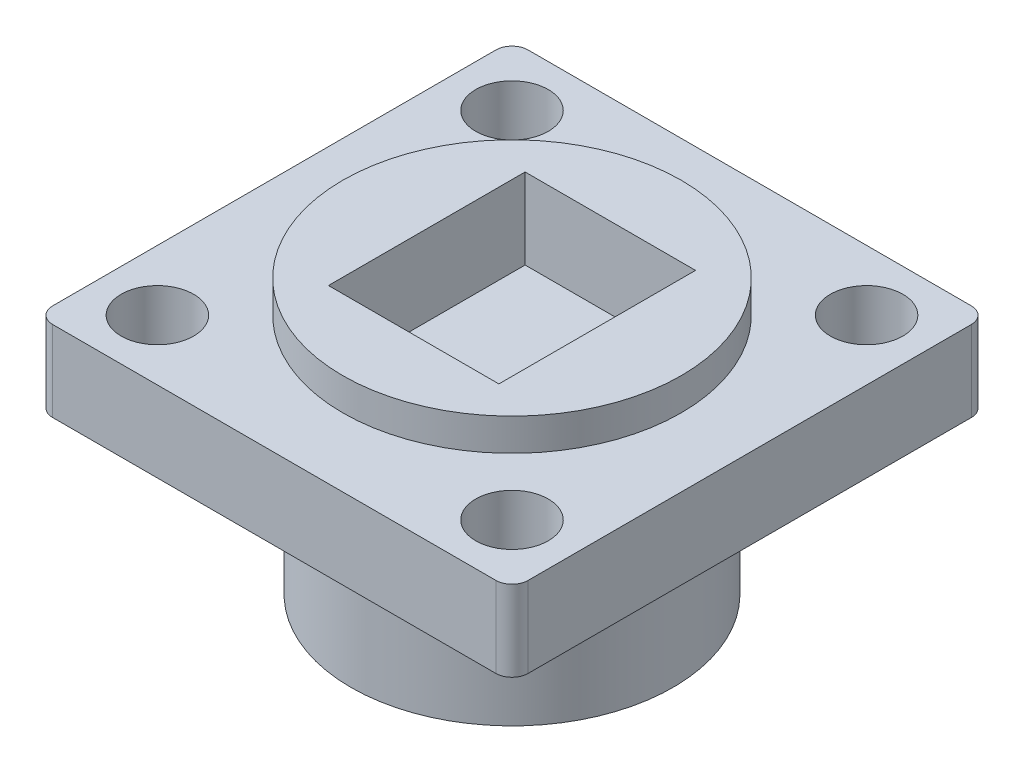
SolidWorks part; units mm, degrees
ref_plane "前视基准面" through (0, 0, 0) normal (0, 0, 1) x (1, 0, 0)
ref_plane "上视基准面" through (0, 0, 0) normal (0, 1, 0) x (1, 0, 0)
ref_plane "右视基准面" through (0, 0, 0) normal (1, 0, 0) x (0, 0, -1)
sketch "草图1" plane through (0, 0, 0) normal (0, 1, 0) x (1, 0, 0)
  circle A0 centre (0, 0) radius 10
  dimension "D1" = 20
extrude "凸台-拉伸1" add sketch "草图1" along normal blind 10
sketch "草图2" plane through (0, 10, 0) normal (0, 1, 0) x (1, 0, 0)
  line L1 (-14.75, 14.75) -> (14.75, 14.75)
  line L2 (-14.75, 14.75) -> (-14.75, -14.75)
  line L3 (-14.75, -14.75) -> (14.75, -14.75)
  line L4 (14.75, 14.75) -> (14.75, -14.75)
  line L5 (-14.75, 14.75) -> (14.75, -14.75) construction
  line L6 (-14.75, -14.75) -> (14.75, 14.75) construction
  point P0 (0, 0)
  dimension "D1" = 29.5
extrude "凸台-拉伸2" add sketch "草图2" along normal blind 5
sketch "草图3" plane through (0, 15, 0) normal (0, 1, 0) x (1, 0, 0)
  circle A0 centre (0, 0) radius 10.5
  dimension "D1" = 21
extrude "凸台-拉伸3" add sketch "草图3" along normal blind 17
sketch "草图4" plane through (0, 15, 0) normal (0, 1, 0) x (1, 0, 0)
  line L1 (-11, 11) -> (11, 11) construction
  line L2 (-11, 11) -> (-11, -11) construction
  line L3 (-11, -11) -> (11, -11) construction
  line L4 (11, 11) -> (11, -11) construction
  line L5 (-11, 11) -> (11, -11) construction
  line L6 (-11, -11) -> (11, 11) construction
  circle A0 centre (11, 11) radius 2.25
  circle A1 centre (-11, 11) radius 2.25
  circle A2 centre (-11, -11) radius 2.25
  circle A3 centre (11, -11) radius 2.25
  point P0 (0, 0)
  dimension "D2" = 4.5
  dimension "D1" = 22
extrude "切除-拉伸1" cut sketch "草图4" against normal blind 17
fillet "圆角1" radius 1 4 edges at (-14.75, 12.5, -14.75) (14.75, 12.5, -14.75) (14.75, 12.5, 14.75) (-14.75, 12.5, 14.75)
sketch "草图5" plane through (0, 32, 0) normal (0, 1, 0) x (1, 0, 0)
  circle A1 centre (0, 0) radius 10.5
  circle A2 centre (0, 0) radius 10.5
  dimension "D1" = 0
extrude "切除-拉伸2" cut sketch "草图5" against normal blind 15
sketch "草图6" plane through (0, 17, 0) normal (0, 1, 0) x (1, 0, 0)
  line L1 (-5.2873, 6.1007) -> (5.2873, 6.1007)
  line L2 (-5.2873, 6.1007) -> (-5.2873, -6.1007)
  line L3 (-5.2873, -6.1007) -> (5.2873, -6.1007)
  line L4 (5.2873, 6.1007) -> (5.2873, -6.1007)
  line L5 (-5.2873, 6.1007) -> (5.2873, -6.1007) construction
  line L6 (-5.2873, -6.1007) -> (5.2873, 6.1007) construction
  point P0 (0, 0)
extrude "切除-拉伸3" cut sketch "草图6" against normal blind 5
